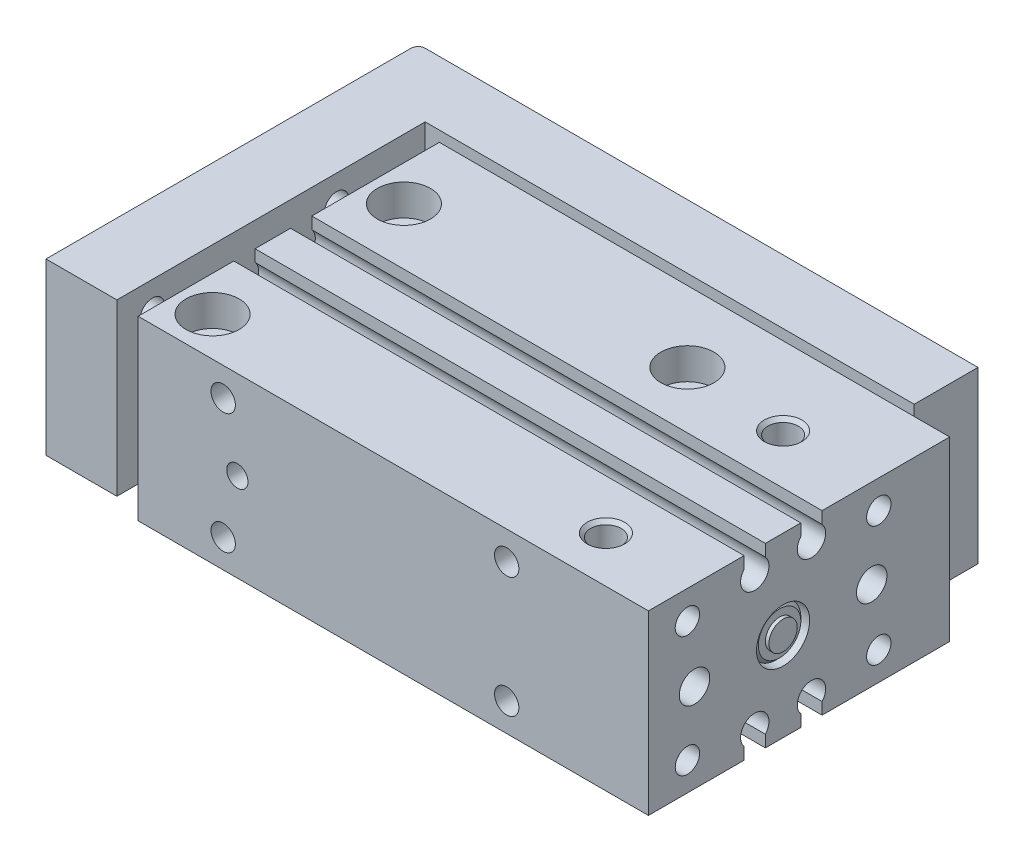
SolidWorks part; units mm, degrees
ref_plane "前视基准面" through (0, 0, 0) normal (0, 0, 1) x (1, 0, 0)
ref_plane "上视基准面" through (0, 0, 0) normal (0, 1, 0) x (1, 0, 0)
ref_plane "右视基准面" through (0, 0, 0) normal (1, 0, 0) x (0, 0, -1)
sketch "草图2" plane through (0, 0, 0) normal (0, 1, 0) x (1, 0, 0)
  line L0 (1, 34.5) -> (79, 34.5)
  line L1 (0, 33.5) -> (0, -18)
  line L2 (0, -18) -> (10, -18)
  line L3 (10, -18) -> (10, 25.5)
  line L4 (10, 25.5) -> (79, 25.5)
  line L5 (79, 25.5) -> (79, 34.5)
  line L6 (0, 0) -> (50000, 0) construction
  arc A0 (1, 34.5) -> (0, 33.5) centre (1, 33.5) ccw
  point P9 (0, 34.5)
  dimension "D1" = 1
  dimension "D2" = 52.5
  dimension "D3" = 78
  dimension "D4" = 9
  dimension "D5" = 10
  dimension "D6" = 34.5
extrude "凸台-拉伸1" add sketch "草图2" along normal mid plane 24
sketch "草图3" plane through (0, 0, 0) normal (0, 1, 0) x (1, 0, 0)
  line L0 (79, 34.5) -> (1, 34.5) construction
  line L1 (14, 23.5) -> (86, 23.5)
  line L2 (14, 23.5) -> (14, -19)
  line L3 (14, -19) -> (86, -19)
  line L4 (86, 23.5) -> (86, -19)
  line L5 (0, 33.5) -> (0, -18) construction
  line L6 (10, 25.5) -> (79, 25.5) construction
  dimension "D1" = 53.5
  dimension "D2" = 86
  dimension "D3" = 14
  dimension "D4" = 2
extrude "凸台-拉伸2" add sketch "草图3" along normal mid plane 25 separate body
sketch "草图5" plane through (86, 0, 0) normal (1, 0, 0) x (0, 0, -1)
  line L0 (0, 0) -> (0, -50000) construction
  line L1 (0, 0) -> (50000, 0) construction
  line L2 (-4, 5.4361) -> (-4, -49994.5639) construction
  line L3 (-5.5, 10.8229) -> (-5.5, 12.5)
  line L4 (-19, 12.5) -> (23.5, 12.5) construction
  line L5 (-5.5, 12.5) -> (-2.5, 12.5)
  line L6 (-2.5, 10.8229) -> (-2.5, 12.5)
  line L7 (-2.5, -10.8229) -> (-2.5, -12.5)
  line L8 (-5.5, -12.5) -> (-2.5, -12.5)
  line L9 (-5.5, -10.8229) -> (-5.5, -12.5)
  line L10 (5.5, -10.8229) -> (5.5, -12.5)
  line L11 (5.5, -12.5) -> (2.5, -12.5)
  line L12 (2.5, -10.8229) -> (2.5, -12.5)
  line L13 (2.5, 10.8229) -> (2.5, 12.5)
  line L14 (5.5, 12.5) -> (2.5, 12.5)
  line L15 (5.5, 10.8229) -> (5.5, 12.5)
  arc A0 (-5.5, 10.8229) -> (-2.5, 10.8229) centre (-4, 9.5) ccw
  arc A1 (-5.5, -10.8229) -> (-2.5, -10.8229) centre (-4, -9.5) cw
  arc A2 (5.5, -10.8229) -> (2.5, -10.8229) centre (4, -9.5) ccw
  arc A3 (5.5, 10.8229) -> (2.5, 10.8229) centre (4, 9.5) cw
  dimension "D2" = 4
  dimension "D1" = 3
  dimension "D3" = 3
  dimension "D4" = 4
extrude "切除-拉伸1" cut sketch "草图5" against normal up to next (72 mm away)
sketch "草图6" plane through (86, 0, 0) normal (1, 0, 0) x (0, 0, -1)
  line L0 (0, 0) -> (50000, 0) construction
  line L1 (0, 0) -> (0, -50000) construction
  circle A0 centre (-13.5, 8.5) radius 1.72
  circle A1 centre (-13.5, -8.5) radius 1.72
  circle A2 centre (13.5, -8.5) radius 1.72
  circle A3 centre (13.5, 8.5) radius 1.72
  dimension "D1" = 3.44
  dimension "D2" = 17
  dimension "D3" = 27
extrude "切除-拉伸2" cut sketch "草图6" against normal blind 6
cosmetic thread "装饰螺纹线1" parameters "D2"=4
cosmetic thread "装饰螺纹线2" parameters "D2"=4
cosmetic thread "装饰螺纹线3" parameters "D2"=4
cosmetic thread "装饰螺纹线4" parameters "D2"=4
sketch "草图7" plane through (86, 0, 0) normal (1, 0, 0) x (0, 0, -1)
  line L0 (0, 0) -> (50000, 0) construction
  line L1 (0, 0) -> (0, -50000) construction
  circle A0 centre (-12.5, 0) radius 2.15
  circle A1 centre (12.5, 0) radius 2.15
  dimension "D1" = 4.3
  dimension "D2" = 25
extrude "切除-拉伸3" cut sketch "草图7" against normal blind 10
cosmetic thread "装饰螺纹线5" parameters "D2"=5
cosmetic thread "装饰螺纹线6" parameters "D2"=5
sketch "草图8" plane through (0, 12.5, 0) normal (0, 1, 0) x (1, 0, 0)
  line L0 (0, 0) -> (50000, 0) construction
  line L1 (14, -5.5) -> (14, -19) construction
  circle A0 centre (19, 13.5) radius 2.15
  circle A1 centre (59, 13.5) radius 2.15
  circle A3 centre (19, -13.5) radius 2.15
  dimension "D2" = 4.3
  dimension "D1" = 27
  dimension "D3" = 5
  dimension "D4" = 40
extrude "切除-拉伸4" cut sketch "草图8" against normal up to next (25 mm away)
cosmetic thread "装饰螺纹线9" parameters "D2"=5
cosmetic thread "装饰螺纹线10" parameters "D2"=5
cosmetic thread "装饰螺纹线11" parameters "D2"=5
sketch "草图9" plane through (0, 12.5, 0) normal (0, 1, 0) x (1, 0, 0)
  line L0 (0, 0) -> (50000, 0) construction
  line L1 (86, -19) -> (86, -5.5) construction
  line L2 (14, -19) -> (86, -19) construction
  circle A0 centre (73.5, 12.5) radius 2.15
  circle A1 centre (73.5, -12.5) radius 2.15
  dimension "D1" = 4.3
  dimension "D2" = 12.5
  dimension "D3" = 6.5
extrude "切除-拉伸5" cut sketch "草图9" against normal blind 4
cosmetic thread "装饰螺纹线7" parameters "D2"=5
cosmetic thread "装饰螺纹线8" parameters "D2"=5
sketch "草图10" plane through (0, 12.5, 0) normal (0, 1, 0) x (1, 0, 0)
  circle A0 centre (19, 13.5) radius 3.75
  circle A1 centre (59, 13.5) radius 3.75
  circle A2 centre (19, -13.5) radius 3.75
  dimension "D1" = 7.5
extrude "切除-拉伸6" cut sketch "草图10" against normal blind 4.4
mirror "镜向1" about plane through (0, 0, 0) normal (0, 1, 0) of "切除-拉伸5", "切除-拉伸6"
chamfer "倒角2" distance 0.5 angle 45 4 edges at (73.5, -12.5, 10.35) (73.5, -12.5, -10.35) (73.5, 12.5, 10.35) (73.5, 12.5, -10.35)
sketch "草图11" plane through (0, 0, 19) normal (0, 0, 1) x (1, 0, 0)
  line L0 (0, 0) -> (50000, 0) construction
  line L1 (14, 12.5) -> (14, -12.5) construction
  circle A0 centre (26, 8.5) radius 1.72
  circle A1 centre (66, 8.5) radius 1.72
  circle A2 centre (66, -8.5) radius 1.72
  circle A3 centre (26, -8.5) radius 1.72
  circle A4 centre (28, 0) radius 1.5
  dimension "D2" = 3.44
  dimension "D5" = 3
  dimension "D1" = 17
  dimension "D3" = 12
  dimension "D4" = 40
  dimension "D6" = 14
extrude "切除-拉伸7" cut sketch "草图11" against normal blind 6
cosmetic thread "装饰螺纹线12" parameters "D2"=4
cosmetic thread "装饰螺纹线13" parameters "D2"=4
cosmetic thread "装饰螺纹线14" parameters "D2"=4
cosmetic thread "装饰螺纹线15" parameters "D2"=4
sketch "草图12" plane through (0, 0, -34.5) normal (0, 0, -1) x (-1, 0, 0)
  line L0 (0, 0) -> (-50000, 0) construction
  line L1 (0, 12) -> (0, -12) construction
  line L3 (-79, 12) -> (-79, -12) construction
  circle A0 centre (-14, -8) radius 1.72
  circle A1 centre (-44, -8) radius 1.72
  circle A2 centre (-44, 8) radius 1.72
  circle A3 centre (-14, 8) radius 1.72
  circle A4 centre (-73, 4) radius 2.1
  circle A5 centre (-65, 4) radius 2.1
  circle A6 centre (-65, -4) radius 2.1
  circle A7 centre (-73, -4) radius 2.1
  dimension "D1" = 3.44
  dimension "D5" = 4.2
  dimension "D7" = 8
  dimension "D8" = 8
  dimension "D2" = 16
  dimension "D3" = 14
  dimension "D4" = 30
  dimension "D6" = 6
extrude "切除-拉伸8" cut sketch "草图12" against normal blind 9
cosmetic thread "装饰螺纹线16" parameters "D2"=4
cosmetic thread "装饰螺纹线17" parameters "D2"=4
cosmetic thread "装饰螺纹线18" parameters "D2"=4
cosmetic thread "装饰螺纹线19" parameters "D2"=4
sketch "草图14" plane through (0, 0, 0) normal (-1, 0, 0) x (0, 0, 1)
  line L0 (0, 0) -> (-50000, 0) construction
  line L1 (0, 0) -> (0, 50000) construction
  circle A0 centre (13, -8) radius 1.72
  circle A1 centre (13, 8) radius 1.72
  circle A2 centre (-13, -8) radius 1.72
  circle A3 centre (-13, 8) radius 1.72
  dimension "D3" = 3.44
  dimension "D1" = 16
  dimension "D2" = 26
extrude "切除-拉伸9" cut sketch "草图14" against normal blind 10
cosmetic thread "装饰螺纹线20" parameters "D2"=4
cosmetic thread "装饰螺纹线21" parameters "D2"=4
cosmetic thread "装饰螺纹线22" parameters "D2"=4
cosmetic thread "装饰螺纹线23" parameters "D2"=4
sketch "草图15" plane through (0, 0, -34.5) normal (0, 0, 1) x (1, 0, 0)
  line L0 (0, 0) -> (50000, 0) construction
  circle A0 centre (64, 8) radius 1.72
  circle A2 centre (44, 8) radius 1.72 construction
  circle A3 centre (64, -8) radius 1.72
  dimension "D1" = 3.44
  dimension "D3" = 20
  dimension "D2" = 16
extrude "切除-拉伸11" cut sketch "草图15" along normal blind 9
cosmetic thread "装饰螺纹线24" parameters "D2"=4
cosmetic thread "装饰螺纹线25" parameters "D2"=4
sketch "草图16" plane through (10, 0, 0) normal (1, 0, 0) x (0, 0, -1)
  circle A0 centre (0, 0) radius 2.5
  dimension "D1" = 5
extrude "凸台-拉伸3" add sketch "草图16" along normal up to next
sketch "草图18" plane through (0, 0, 0) normal (-1, 0, 0) x (0, 0, 1)
  line L0 (-33.5, 12) -> (18, 12) construction
  line L1 (3, -12) -> (-3, -12)
  line L2 (3, -12) -> (3, 12)
  line L3 (3, 12) -> (-3, 12)
  line L4 (-3, -12) -> (-3, 12)
  line L5 (3, -12) -> (-3, 12) construction
  line L6 (3, 12) -> (-3, -12) construction
  circle A0 centre (0, 0) radius 3.75
  point P0 (0, 0)
  dimension "D2" = 7.5
  dimension "D1" = 6
extrude "切除-拉伸12" cut sketch "草图18" against normal through all contours L2 A0 | L4 A0 | L2 A0 L4
sketch "草图21" plane through (10, 0, 0) normal (1, 0, 0) x (0, 0, -1)
  circle A0 centre (0, 0) radius 3.75
  circle A1 centre (0, 0) radius 2
  dimension "D1" = 7.5
  dimension "D2" = 4
extrude "凸台-拉伸5" add sketch "草图21" against normal blind 5 separate body
sketch "草图17" plane through (10, 0, 0) normal (1, 0, 0) x (0, 0, -1)
  line L0 (0, 0) -> (0, -50000) construction
  line L2 (3.4641, 0) -> (1.7321, 3)
  line L3 (1.7321, 3) -> (-1.7321, 3)
  line L4 (-1.7321, 3) -> (-3.4641, 0)
  line L5 (-3.4641, 0) -> (-1.7321, -3)
  line L6 (-1.7321, -3) -> (1.7321, -3)
  line L7 (1.7321, -3) -> (3.4641, 0)
  circle A0 centre (0, 0) radius 3 construction
  circle A1 centre (0, 0) radius 2
  dimension "D2" = 4
  dimension "D1" = 6
extrude "凸台-拉伸4" add sketch "草图17" along normal blind 2 and the other way blind 10
sketch "草图19" plane through (0, 0, 0) normal (0, 1, 0) x (1, 0, 0)
  line L0 (20.7772, 0) -> (-14.4624, 0) construction
  line L1 (11.7321, 3.4641) -> (12, 3)
  line L2 (12, 3.4641) -> (11.7321, 3.4641)
  line L3 (12, 3.4641) -> (12, 3)
  line L4 (6, 9.2492) -> (6, -9.0078) construction
  line L7 (0, 3.4641) -> (0, 3)
  line L8 (0, 3.4641) -> (0.2679, 3.4641)
  line L9 (0.2679, 3.4641) -> (0, 3)
  line L14 (0, 33.5) -> (0, -18) construction
  line L16 (12, 1.7321) -> (12, -1.7321) construction
  dimension "D1" = 6
  dimension "D2" = 30
revolve "切除-旋转1" cut sketch "草图19" angle 360 about L0
sketch "草图20" plane through (0, 0, 0) normal (0, 0, 1) x (1, 0, 0)
  line L0 (86, 12.5) -> (86, -12.5) construction
  line L1 (0, 0) -> (86, 0)
  line L2 (0, 0) -> (0, 2)
  line L3 (0, 2) -> (14, 2)
  line L4 (86, 0) -> (86, 2)
  line L5 (0, 1.5) -> (0.5, 2)
  line L6 (14, 3) -> (14.5, 3.5)
  line L7 (14, 12.5) -> (14, -12.5) construction
  line L9 (14, 2) -> (14, 3)
  line L10 (14.5, 3.5) -> (85, 3.5)
  line L11 (85.5, 2) -> (85.5, 3)
  line L12 (85.5, 3) -> (85, 3.5)
  line L13 (85.5, 2) -> (86, 2)
  point P12 (85.5, 3.5)
  point P13 (14, 3.5)
  dimension "D1" = 2
  dimension "D2" = 0.5
  dimension "D3" = 45
  dimension "D4" = 0.5
  dimension "D6" = 1.5
revolve "旋转1" add sketch "草图20" angle 360 about L1
